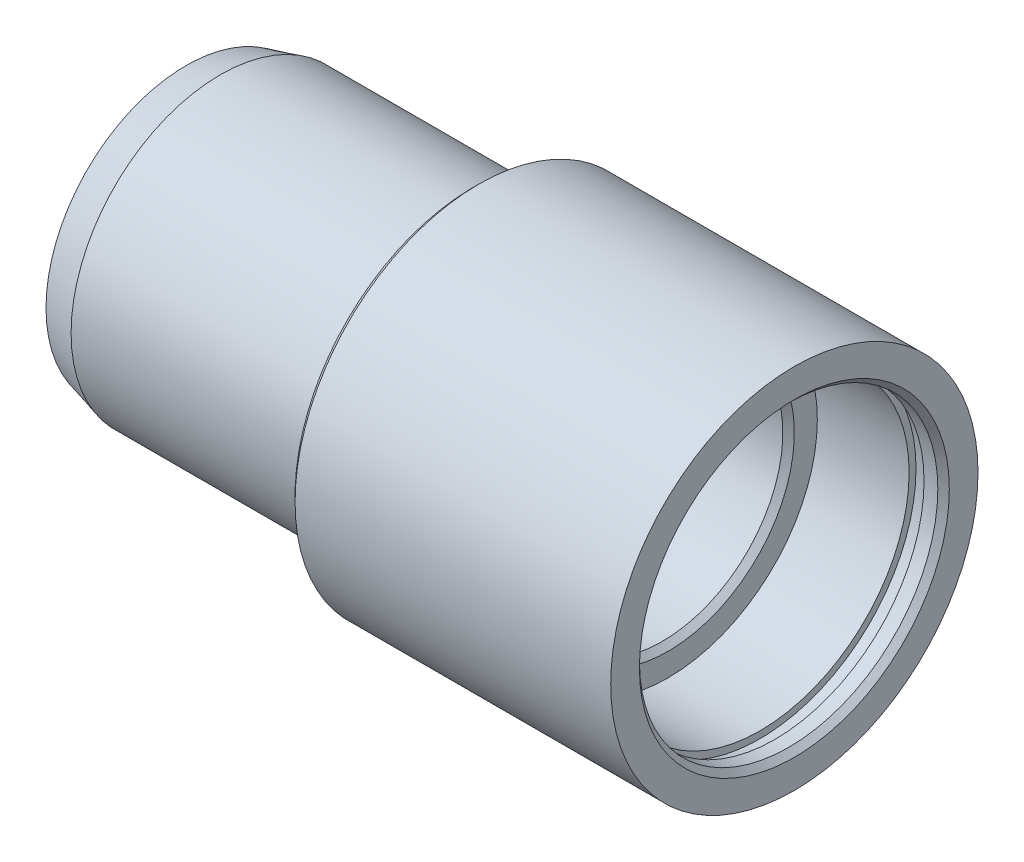
from build123d import *

# Parameters (mm, degrees)
CHAMFER_1_SIZE = 0.5


with BuildPart() as part:
    # 草图1 → 旋转1 (revolve)
    with BuildSketch(Plane(origin=(0, 0, 0), x_dir=(1, 0, 0), z_dir=(0, 1, 0)), mode=Mode.PRIVATE) as revolve_1_sk:
        Polygon((-28.614259258, 10.5), (13.385740742, 10.5), (13.385740742, 13), (21.385740742, 13), (21.385740742, 13.6), (22.685740742, 13.6), (22.685740742, 13), (24.385740742, 13), (24.385740742, 16), (-3.614259258, 16), (-3.614259258, 13), (-25.628618612, 13), (-28.614259258, 12.2), align=None)
    revolve(revolve_1_sk.sketch.rotate(Axis((0, 0, 0), (1, 0, 0)), 180), axis=Axis((0, 0, 0), (1, 0, 0)))

    # 倒角1
    chamfer_1_edges = [part.edges().sort_by_distance(p)[0] for p in [
        (-3.614259258, 0, -16),
        (24.385740742, 0, -13),
        (13.385740742, 0, -10.5),
        (-28.614259258, 0, -10.5),
    ]]
    chamfer(chamfer_1_edges, length=CHAMFER_1_SIZE)


solid = part.part
